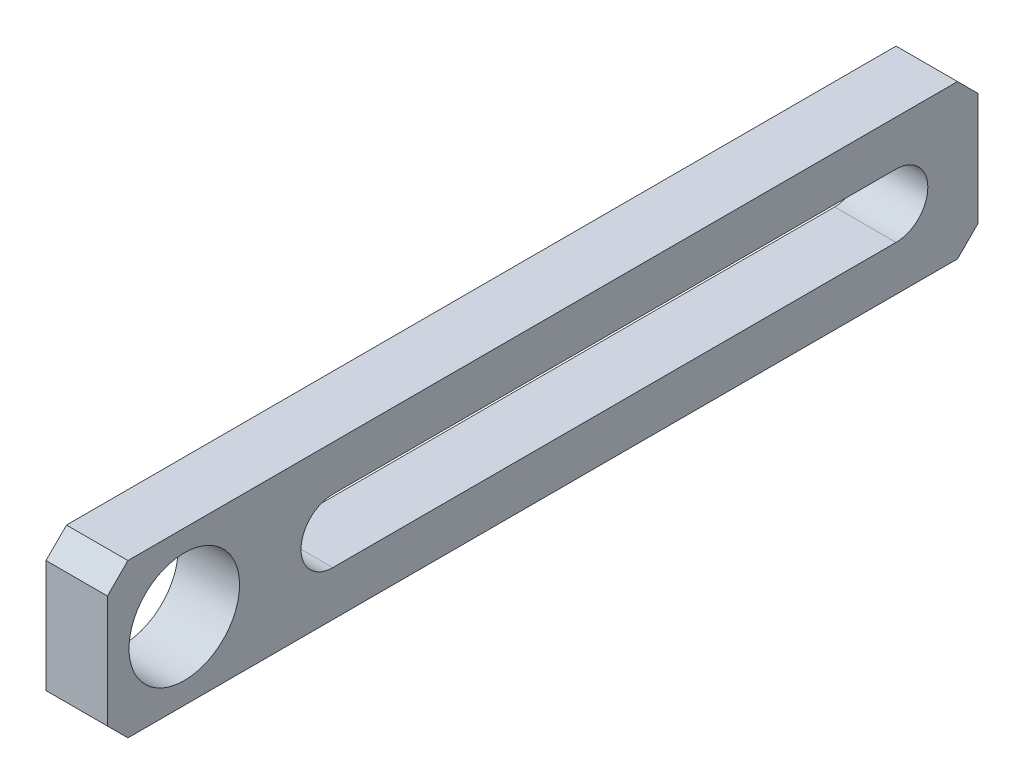
from build123d import *

# Parameters (mm, degrees)
SKETCH1_W              = 85
SKETCH1_H              = 15
EXTRUDE1_DEPTH         = 6
M12X1_0_TAPPED_HOLE1_D = 10.8
CHAMFER1_SIZE          = 2


with BuildPart() as part:
    # Sketch1 → Extrude1 (new body)
    with BuildSketch(Plane(origin=(0, 0, 0), x_dir=(0, 0, -1), z_dir=(1, 0, 0))):
        with Locations((42.5, -7.5)):
            Rectangle(SKETCH1_W, SKETCH1_H)
        with BuildLine():
            Line((22, -4.4), (77, -4.4))
            ThreePointArc((77, -4.4), (80.1, -7.5), (77, -10.6))
            Line((77, -10.6), (22, -10.6))
            ThreePointArc((22, -10.6), (18.9, -7.5), (22, -4.4))
        make_face(mode=Mode.SUBTRACT)
    extrude(amount=EXTRUDE1_DEPTH)

    # M12x1.0 Tapped Hole1 (through all)
    with Locations(Plane(origin=(6, 0, 0), x_dir=(0, 0, -1), z_dir=(1, 0, 0))):
        with Locations((7.5, -7.5)):
            Hole(M12X1_0_TAPPED_HOLE1_D / 2)

    # Chamfer1
    chamfer1_edges = [part.edges().sort_by_distance(p)[0] for p in [
        (3, 0, 0),
        (3, 0, -85),
        (3, -15, -85),
        (3, -15, 0),
    ]]
    chamfer(chamfer1_edges, length=CHAMFER1_SIZE)


solid = part.part
